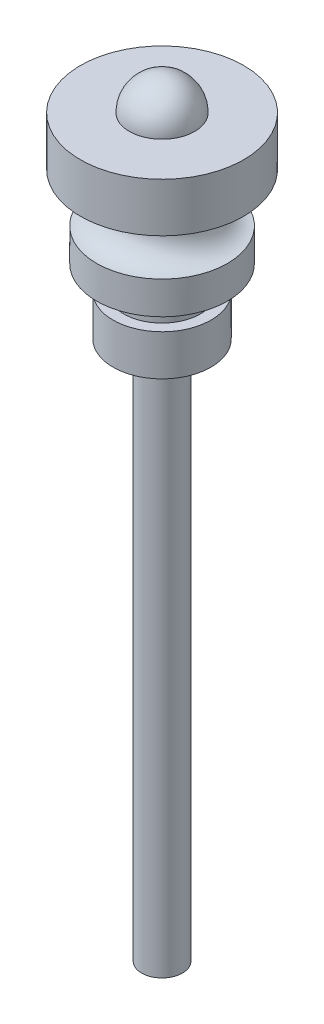
SolidWorks part; units mm, degrees
ref_plane "Front Plane" through (0, 0, 0) normal (0, 0, 1) x (1, 0, 0)
ref_plane "Top Plane" through (0, 0, 0) normal (0, 1, 0) x (1, 0, 0)
ref_plane "Right Plane" through (0, 0, 0) normal (1, 0, 0) x (0, 0, -1)
sketch "Sketch1" plane through (0, 0, 0) normal (0, 0, 1) x (1, 0, 0)
  line L0 (0, 0) -> (10, 0)
  line L1 (10, 0) -> (10, -6)
  line L2 (10, -6) -> (8, -6)
  line L3 (8, -6) -> (8, -16)
  line L4 (8, -16) -> (4.7, -16)
  line L5 (4.7, -16) -> (4.7, -19)
  line L6 (4.7, -19) -> (6, -19)
  line L7 (6, -19) -> (6, -24)
  line L8 (6, -24) -> (2.5, -24)
  line L9 (2.5, -24) -> (2.5, -90)
  line L10 (2.5, -90) -> (0, -90)
  line L11 (0, -90) -> (0, 0)
  line L12 (0, 0) -> (0, 5.4429) construction
  point P14 (4.25, -24)
  dimension "D1" = 20
  dimension "D2" = 16
  dimension "D3" = 5
  dimension "D4" = 12
  dimension "D5" = 9.4
  dimension "D6" = 6
  dimension "D7" = 8
  dimension "D8" = 24
  dimension "D9" = 3
  dimension "D10" = 90
revolve "Revolve1" add sketch "Sketch1" angle 360 about L12
sketch "Sketch2" plane through (0, 0, 0) normal (0, 0, 1) x (1, 0, 0)
  line L0 (0, 5.1057) -> (0, -21.4611) construction
  line L1 (-8, -6) -> (8, -6) construction
  line L2 (8, -6) -> (17.8139, -6)
  line L3 (17.8139, -6) -> (17.8139, -12)
  line L4 (17.8139, -12) -> (8, -12)
  line L5 (-8, -16) -> (8, -16) construction
  arc A0 (8, -6) -> (8, -12) centre (8, -9) ccw
  point P5 (5, -9)
  dimension "D1" = 4
  dimension "D2" = 5
revolve "Cut-Revolve1" cut sketch "Sketch2" angle 360 about L0
sketch "Sketch4" plane through (0, 0, 0) normal (0, 0, 1) x (1, 0, 0)
  line L0 (0, 4) -> (0, 0)
  line L1 (0, 0) -> (4, 0)
  arc A0 (4, 0) -> (0, 4) centre (0, 0) ccw
  dimension "D1" = 8
revolve "Revolve3" add sketch "Sketch4" angle 360 about L0
